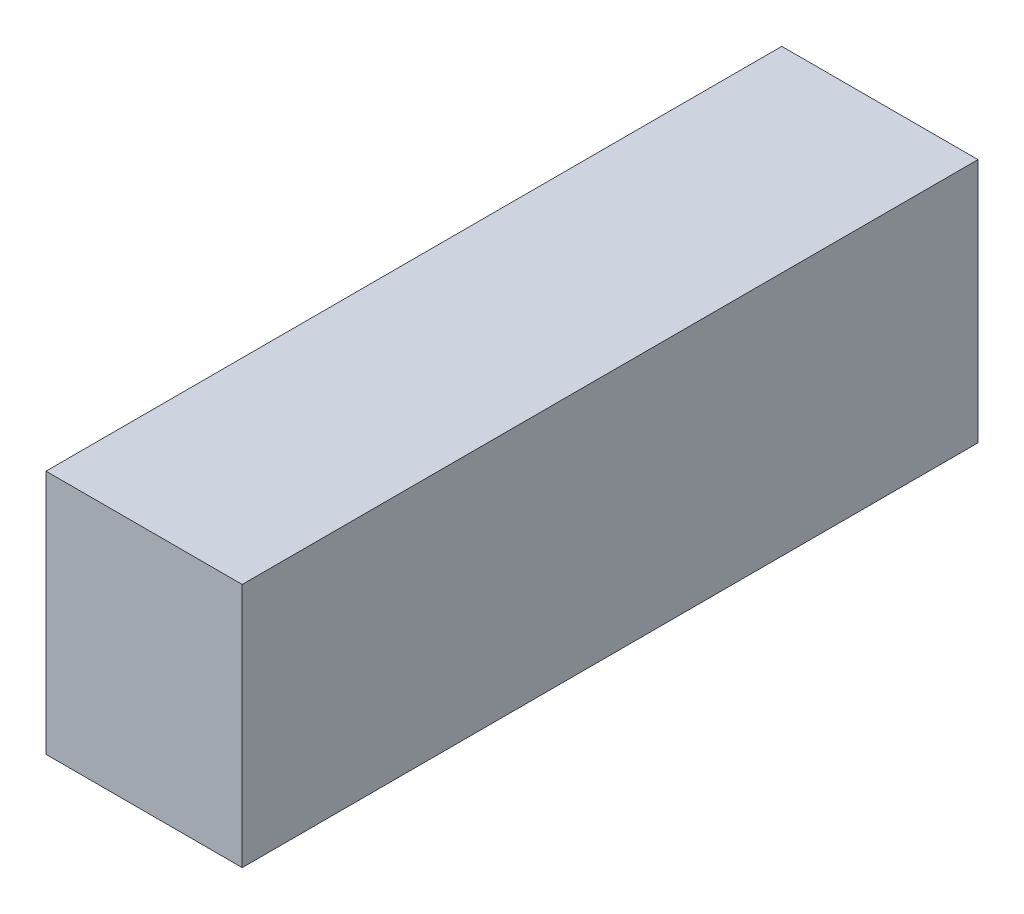
SolidWorks part; units mm, degrees
ref_plane "Front Plane" through (0, 0, 0) normal (0, 0, 1) x (1, 0, 0)
ref_plane "Top Plane" through (0, 0, 0) normal (0, 1, 0) x (1, 0, 0)
ref_plane "Right Plane" through (0, 0, 0) normal (1, 0, 0) x (0, 0, -1)
sketch "Sketch1" plane through (0, 0, 0) normal (0, 1, 0) x (1, 0, 0)
  line L3 (-4, 15) -> (4, 15)
  line L4 (-4, 15) -> (-4, -15)
  line L5 (-4, -15) -> (4, -15)
  line L6 (4, 15) -> (4, -15)
  line L7 (-4, 15) -> (4, -15) construction
  line L8 (-4, -15) -> (4, 15) construction
  point P0 (0, 0)
  dimension "D1" = 30
  dimension "D2" = 8
extrude "Boss-Extrude1" add sketch "Sketch1" along normal blind 10
